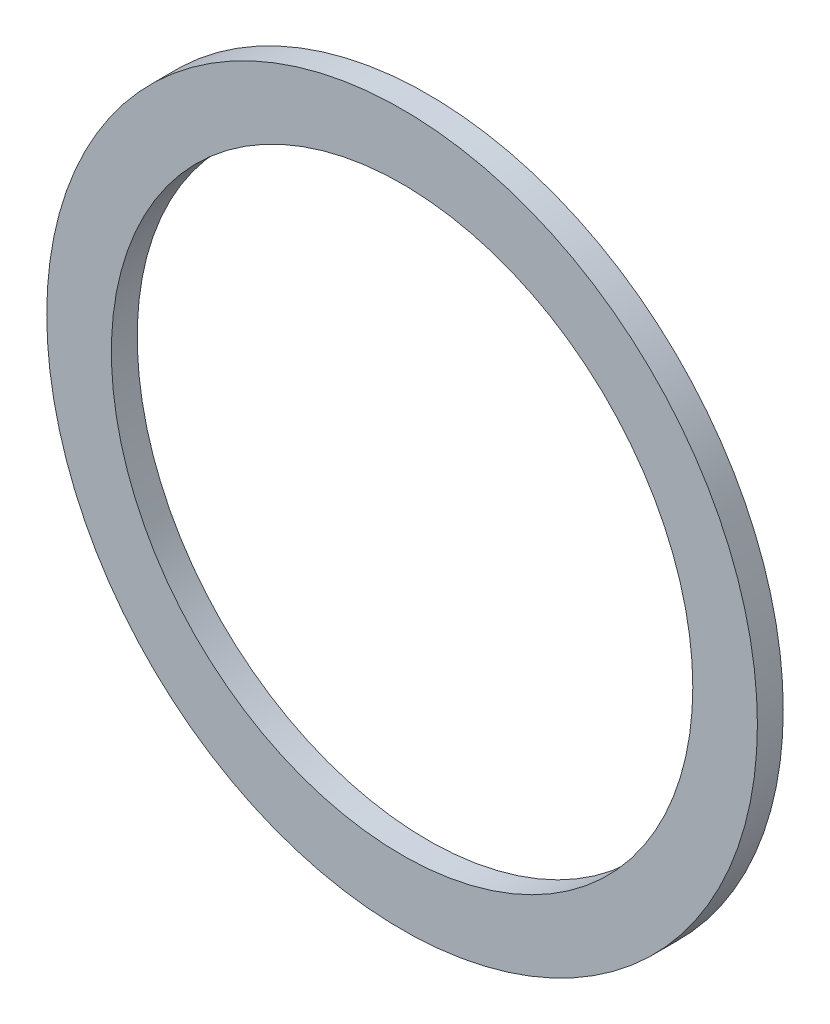
SolidWorks part; units mm, degrees
material "山都平"
ref_plane "前视基准面" through (0, 0, 0) normal (0, 0, 1) x (1, 0, 0)
ref_plane "上视基准面" through (0, 0, 0) normal (0, 1, 0) x (1, 0, 0)
ref_plane "右视基准面" through (0, 0, 0) normal (1, 0, 0) x (0, 0, -1)
sketch "草图1" plane through (0, 0, 0) normal (0, 0, 1) x (1, 0, 0)
  circle A0 centre (0, 0) radius 27.5
  circle A1 centre (0, 0) radius 22.5
  dimension "D1" = 55
  dimension "D2" = 45
extrude "凸台-拉伸1" add sketch "草图1" along normal blind 2
